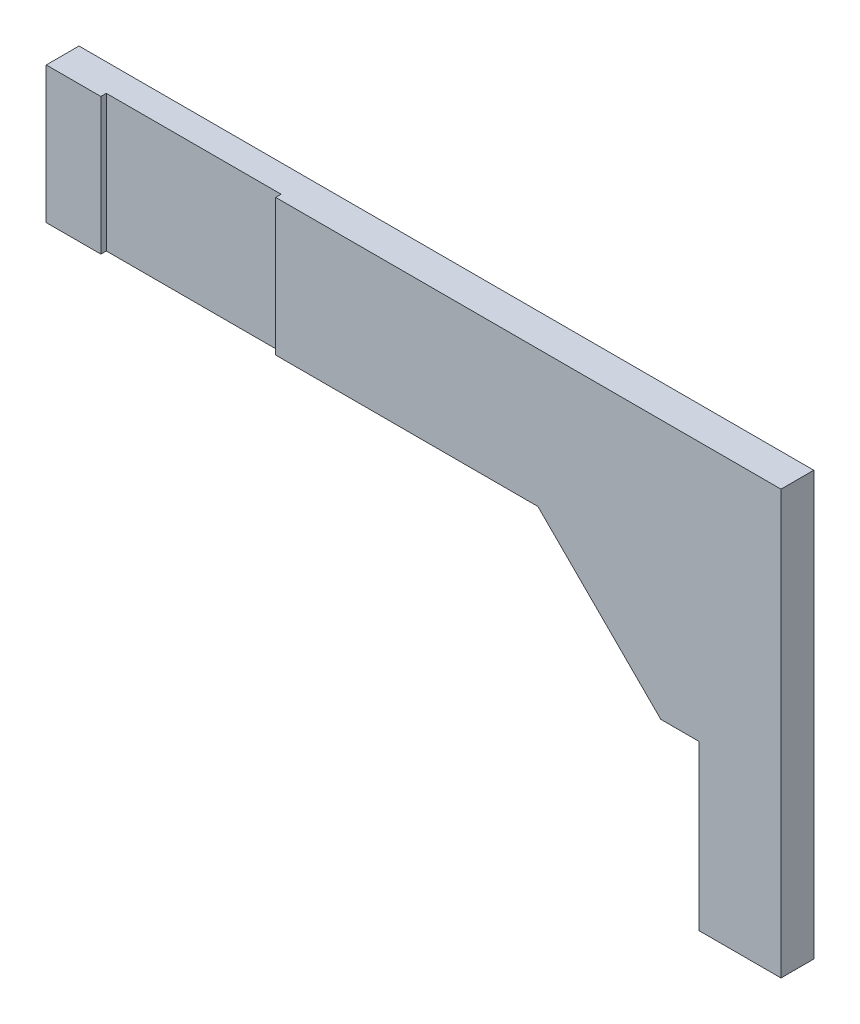
SolidWorks part; units mm, degrees
ref_plane "前视基准面" through (0, 0, 0) normal (0, 0, 1) x (1, 0, 0)
ref_plane "上视基准面" through (0, 0, 0) normal (0, 1, 0) x (1, 0, 0)
ref_plane "右视基准面" through (0, 0, 0) normal (1, 0, 0) x (0, 0, -1)
sketch "草图1" plane through (0, 0, 0) normal (0, 0, 1) x (1, 0, 0)
  line L0 (0, 0) -> (0, 60)
  line L1 (0, 60) -> (-14, 60)
  line L2 (-14, 60) -> (-59, 105)
  line L3 (-59, 105) -> (-239, 105)
  line L4 (-239, 105) -> (-239, 155)
  line L5 (-239, 155) -> (30, 155)
  line L6 (30, 155) -> (30, 0)
  line L8 (0, 0) -> (30, 0)
  dimension "D1" = 14
  dimension "D2" = 60
  dimension "D3" = 45
  dimension "D4" = 50
  dimension "D5" = 30
  dimension "D6" = 180
  dimension "D7" = 45
extrude "凸台-拉伸1" add sketch "草图1" along normal mid plane 12
sketch "草图2" plane through (0, 0, 6) normal (0, 0, -1) x (-1, 0, 0)
  line L0 (-30, 155) -> (239, 155) construction
  line L1 (219, 155) -> (155, 155)
  line L2 (219, 155) -> (219, 105)
  line L3 (219, 105) -> (155, 105)
  line L4 (155, 155) -> (155, 105)
  line L6 (239, 105) -> (59, 105) construction
  line L8 (239, 155) -> (239, 105) construction
  point P6 (0, 0)
  point P7 (0, 0)
  point P10 (0, 0)
  dimension "D1" = 64
  dimension "D2" = 20
extrude "切除-拉伸1" cut sketch "草图2" along normal blind 2
